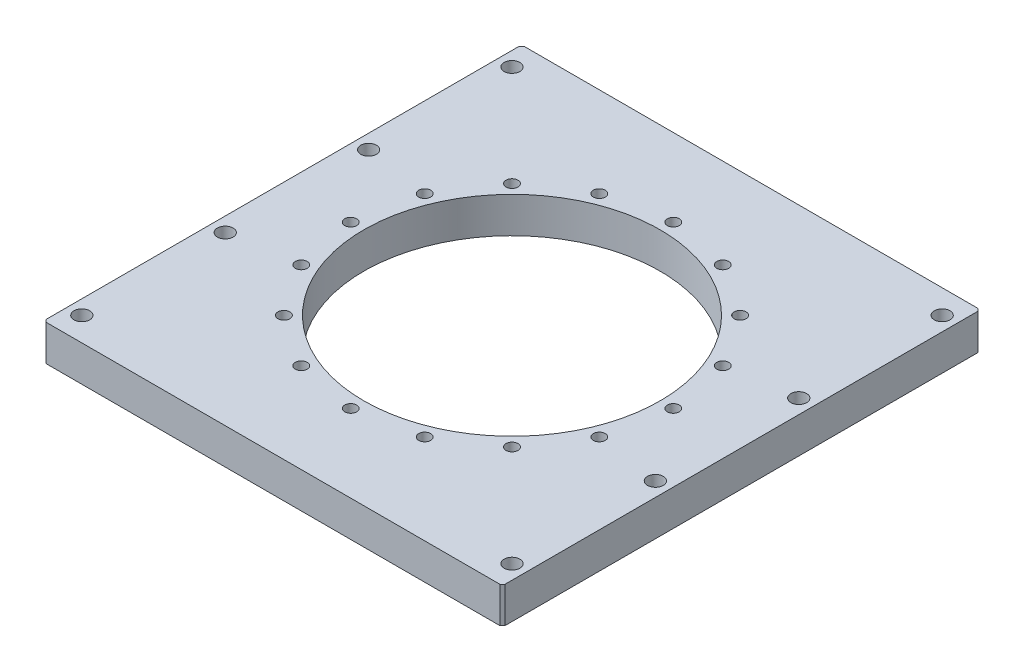
from build123d import *

# Parameters (mm, degrees)
SKETCH_1_W                = 192
SKETCH_1_H                = 200
EXTRUDE_1_DEPTH           = 7.5
CHAMFER_1_SIZE            = 1
HOLE_WIZARD_1_D           = 6.6
HOLE_WIZARD_1_CBORE_D     = 11
HOLE_WIZARD_1_CBORE_DEPTH = 6.8
SKETCH_7_R                = 62
CUT_EXTRUDE_1_DEPTH       = 15
HOLE_WIZARD_M6_1_D        = 5


with BuildPart() as part:
    # 草图1 → 凸台-拉伸1 (new, symmetric)
    with BuildSketch(Plane(origin=(0, 0, 0), x_dir=(1, 0, 0), z_dir=(0, 1, 0))):
        Rectangle(SKETCH_1_W, SKETCH_1_H)
    extrude(amount=EXTRUDE_1_DEPTH, both=True)

    # 倒角1
    chamfer_1_edges = [part.edges().sort_by_distance(p)[0] for p in [
        (96, 0, 100),
        (-96, 0, 100),
        (-96, 0, -100),
        (96, 0, -100),
    ]]
    chamfer(chamfer_1_edges, length=CHAMFER_1_SIZE)

    # 打孔尺寸(%根据)内六角圆柱头螺钉的类型1 (through all)
    with Locations(Plane(origin=(0, -7.5, 0), x_dir=(-1, 0, 0), z_dir=(0, -1, 0))):
        with Locations((90, -90), (90, -30), (-90, -30), (-90, -90), (-90, 90), (-90, 30), (90, 30), (90, 90)):
            CounterBoreHole(HOLE_WIZARD_1_D / 2, HOLE_WIZARD_1_CBORE_D / 2, HOLE_WIZARD_1_CBORE_DEPTH)

    # 草图7 → 切除-拉伸1 (cut)
    with BuildSketch(Plane(origin=(0, 7.5, 0), x_dir=(1, 0, 0), z_dir=(0, 1, 0))):
        with Locations(Location((0, 0, 0), (0, 0, 270))):
            Circle(SKETCH_7_R)
    extrude(amount=-CUT_EXTRUDE_1_DEPTH, mode=Mode.SUBTRACT)

    # M6 螺纹孔1 (through all)
    with Locations(Plane(origin=(0, -7.5, 0), x_dir=(-1, 0, 0), z_dir=(0, -1, 0))):
        with Locations((67.5, 0), (62.361868445, -25.831131685), (47.72970773, -47.72970773), (25.831131685, -62.361868445), (0, -67.5), (-25.831131685, -62.361868445), (-47.72970773, -47.72970773), (-62.361868445, -25.831131685), (-67.5, 0), (-62.361868445, 25.831131685), (-47.72970773, 47.72970773), (-25.831131685, 62.361868445), (0, 67.5), (25.831131685, 62.361868445), (47.72970773, 47.72970773), (62.361868445, 25.831131685)):
            Hole(HOLE_WIZARD_M6_1_D / 2)


solid = part.part
